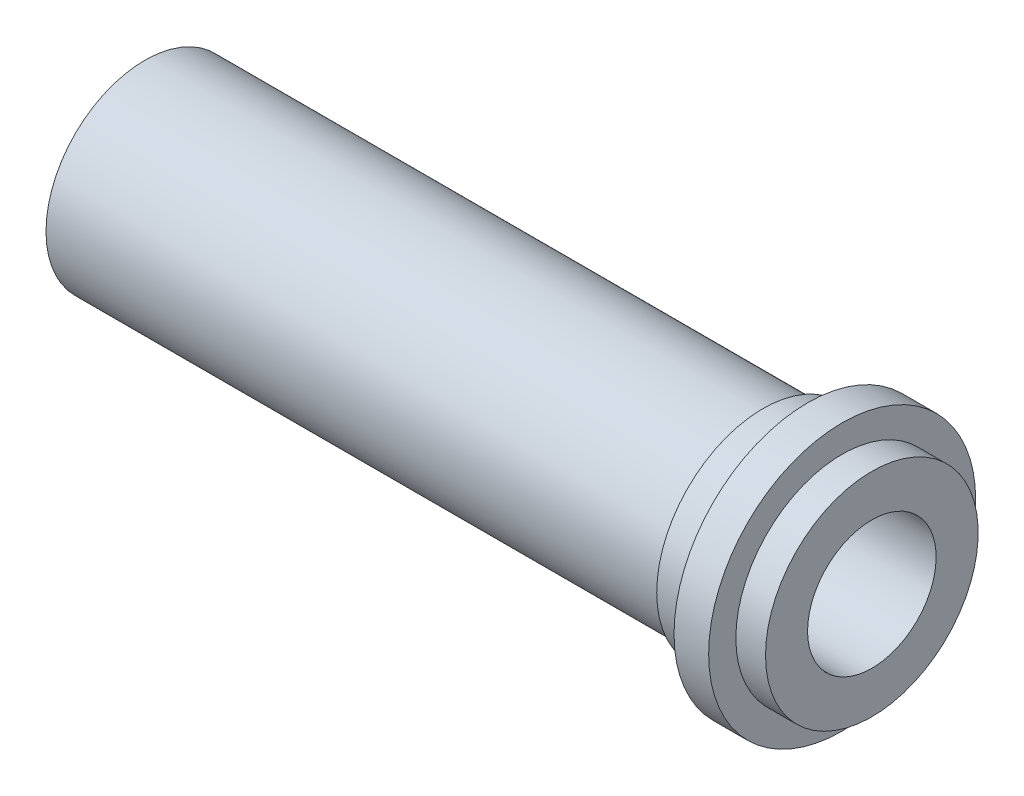
SolidWorks part; units mm, degrees
ref_plane "前视基准面" through (0, 0, 0) normal (0, 0, 1) x (1, 0, 0)
ref_plane "上视基准面" through (0, 0, 0) normal (0, 1, 0) x (1, 0, 0)
ref_plane "右视基准面" through (0, 0, 0) normal (1, 0, 0) x (0, 0, -1)
sketch "草图1" plane through (0, 0, 0) normal (0, 0, 1) x (1, 0, 0)
  line L0 (0, 13) -> (0, 20)
  line L1 (0, 20) -> (125, 20)
  line L2 (125, 20) -> (125, 21.5)
  line L3 (125, 21.5) -> (147, 21.5)
  line L4 (147, 21.5) -> (147, 13)
  line L5 (147, 13) -> (0, 13)
  line L6 (0, 0) -> (68.1552, 0) construction
  dimension "D1" = 20
  dimension "D2" = 7
  dimension "D3" = 22
  dimension "D4" = 125
  dimension "D5" = 1.5
revolve "旋转1" add sketch "草图1" angle 360 about L6
sketch "草图2" plane through (147, 0, 0) normal (1, 0, 0) x (0, 0, -1)
  circle A0 centre (0, 0) radius 27
  circle A1 centre (0, 0) radius 21.5 construction
  circle A2 centre (0, 0) radius 21.5
  dimension "D1" = 54
extrude "凸台-拉伸1" add sketch "草图2" against normal blind 7 from offset 6 offset against normal yes
sketch "草图3" plane through (141, 0, 0) normal (1, 0, 0) x (0, 0, -1)
  circle A0 centre (0, 0) radius 27
  circle A1 centre (0, 0) radius 33.5
  circle A2 centre (0, 0) radius 27 construction
  dimension "D1" = 67
extrude "凸台-拉伸2" [suppressed] add sketch "草图3" along normal blind 15
